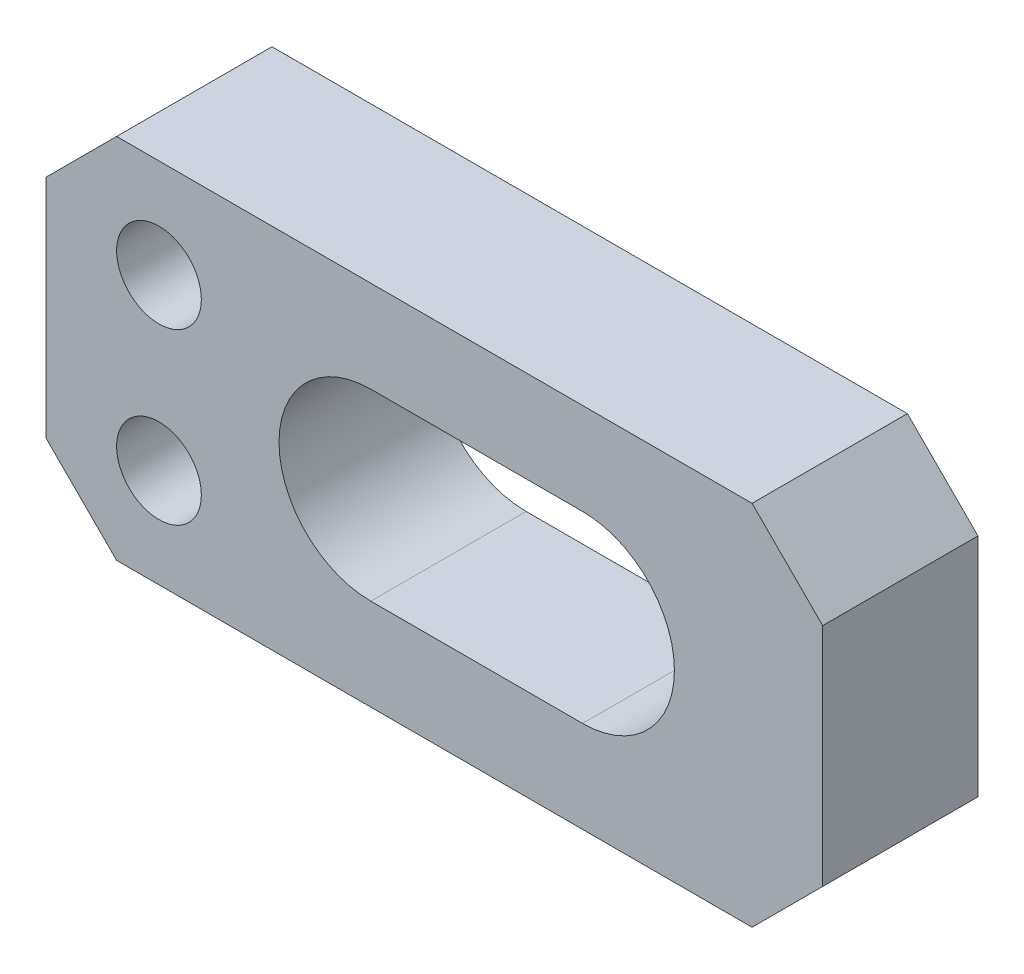
from build123d import *

# Parameters (mm, degrees)
SKETCH_1_W      = 55
SKETCH_1_H      = 26
SKETCH_1_R      = 3
EXTRUDE_1_DEPTH = 11
CHAMFER_1_SIZE  = 5


with BuildPart() as part:
    # 草图1 → 凸台-拉伸1 (new body)
    with BuildSketch(Plane.XY):
        Rectangle(SKETCH_1_W, SKETCH_1_H)
        with Locations((-19.5, 6)):
            Circle(SKETCH_1_R, mode=Mode.SUBTRACT)
        with Locations((-19.5, -6)):
            Circle(SKETCH_1_R, mode=Mode.SUBTRACT)
        with BuildLine():
            Line((-4.5, 6.5), (10.5, 6.5))
            ThreePointArc((10.5, 6.5), (17, 0), (10.5, -6.5))
            Line((10.5, -6.5), (-4.5, -6.5))
            ThreePointArc((-4.5, -6.5), (-11, 0), (-4.5, 6.5))
        make_face(mode=Mode.SUBTRACT)
    extrude(amount=EXTRUDE_1_DEPTH)

    # 倒角1
    chamfer_1_edges = [part.edges().sort_by_distance(p)[0] for p in [
        (27.5, -13, 5.5),
        (-27.5, -13, 5.5),
        (-27.5, 13, 5.5),
        (27.5, 13, 5.5),
    ]]
    chamfer(chamfer_1_edges, length=CHAMFER_1_SIZE)


solid = part.part
